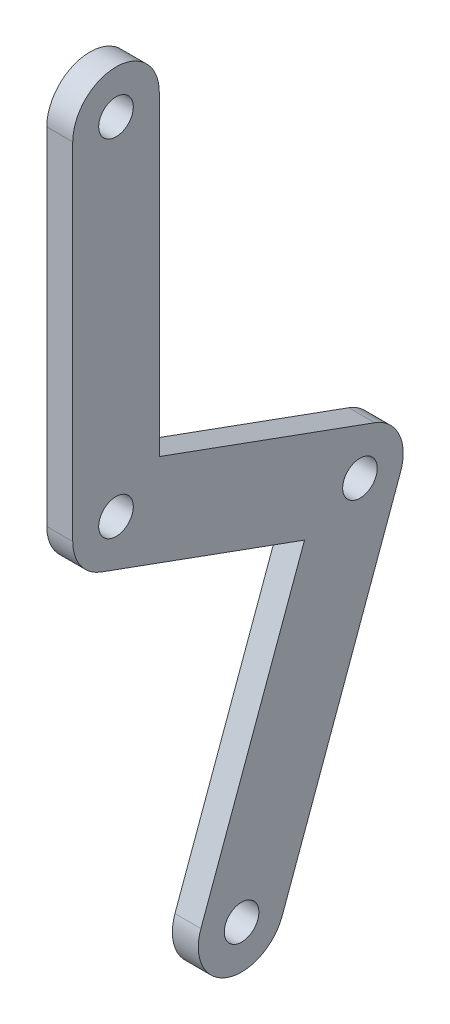
SolidWorks part; units mm, degrees
material "AISI 1045 Steel, cold drawn"
ref_plane "Front Plane" through (0, 0, 0) normal (0, 0, 1) x (1, 0, 0)
ref_plane "Top Plane" through (0, 0, 0) normal (0, 1, 0) x (1, 0, 0)
ref_plane "Right Plane" through (0, 0, 0) normal (1, 0, 0) x (0, 0, -1)
sketch "Sketch1" plane through (0, 0, 0) normal (1, 0, 0) x (0, 0, -1)
  line L0 (0, 0) -> (56.3816, -20.5212) construction
  line L1 (56.3816, -20.5212) -> (29.0199, -95.6966) construction
  line L2 (0, -5.4306) -> (0, 80) construction
  line L3 (0, 55) -> (0, -55) construction
  line L4 (0, 80) -> (0, 0) construction
  line L5 (10, 80) -> (10, 0)
  line L6 (-10, 80) -> (-10, 0)
  line L7 (0, 0) -> (56.3816, -20.5212) construction
  line L8 (3.4202, 9.3969) -> (59.8018, -11.1243)
  line L9 (-3.4202, -9.3969) -> (52.9614, -29.9181)
  line L10 (56.3816, -20.5212) -> (29.0199, -95.6966) construction
  line L11 (65.7785, -23.9414) -> (38.4169, -99.1168)
  line L12 (46.9846, -17.101) -> (19.623, -92.2764)
  arc A0 (10, 80) -> (-10, 80) centre (0, 80) ccw
  arc A1 (-10, 0) -> (10, 0) centre (0, 0) ccw
  arc A2 (3.4202, 9.3969) -> (-3.4202, -9.3969) centre (0, 0) ccw
  arc A3 (52.9614, -29.9181) -> (59.8018, -11.1243) centre (56.3816, -20.5212) ccw
  arc A4 (65.7785, -23.9414) -> (46.9846, -17.101) centre (56.3816, -20.5212) ccw
  arc A5 (19.623, -92.2764) -> (38.4169, -99.1168) centre (29.0199, -95.6966) ccw
  circle A6 centre (0, 80) radius 4
  circle A7 centre (0, 0) radius 4
  circle A8 centre (56.3816, -20.5212) radius 4
  circle A9 centre (29.0199, -95.6966) radius 4
  point P7 (0, 40)
  point P12 (28.1908, -10.2606)
  point P18 (42.7008, -58.1089)
  dimension "D6" = 10
  dimension "D7" = 8
  dimension "D1" = 80
  dimension "D2" = 60
  dimension "D3" = 80
  dimension "D4" = 110
  dimension "D5" = 90
extrude "Boss-Extrude1" add sketch "Sketch1" along normal blind 6 contours L12 A5 L11 A3 L9 A9 | A3 A4 L12 L9 A8 | A4 L8 L5 A1 L9 L12 | L8 A2 A1 L5 A7 | A2 L8 L5 A0 L6 A6
